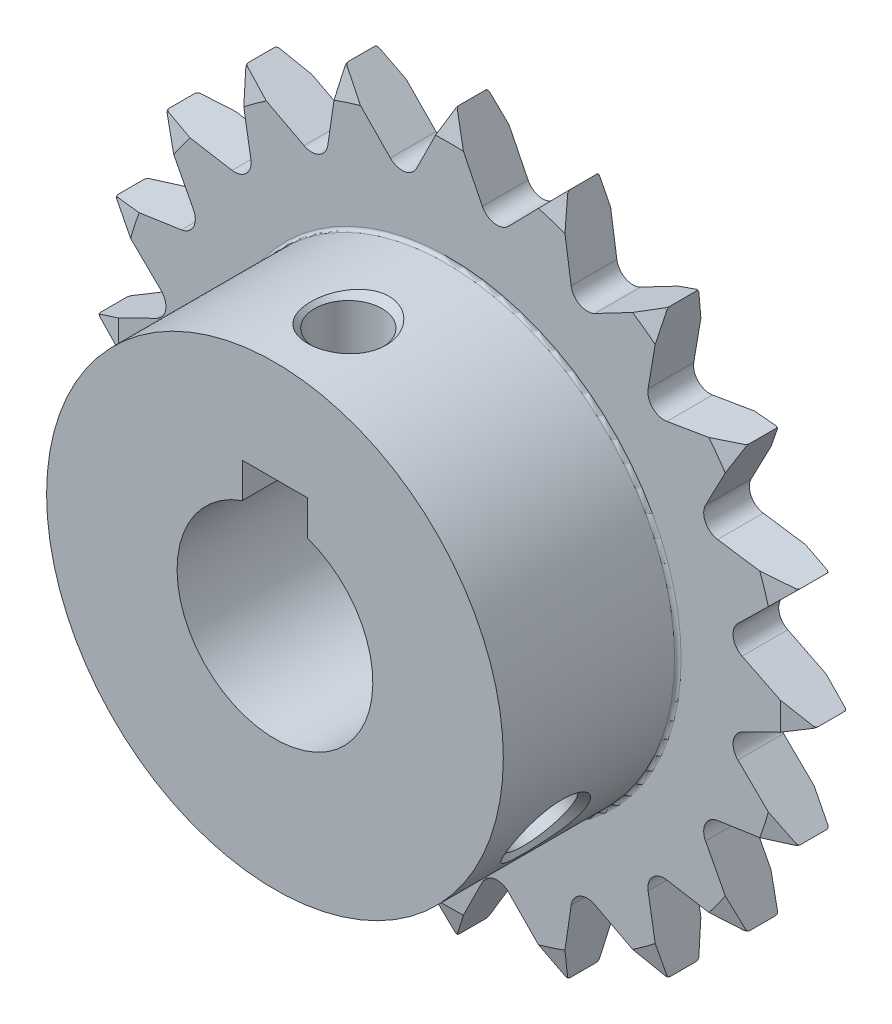
SolidWorks part; units mm, degrees
ref_plane "前视基准面" through (0, 0, 0) normal (0, 0, 1) x (1, 0, 0)
ref_plane "上视基准面" through (0, 0, 0) normal (0, 1, 0) x (1, 0, 0)
ref_plane "右视基准面" through (0, 0, 0) normal (1, 0, 0) x (0, 0, -1)
sketch "草图1" plane through (0, 0, 0) normal (1, 0, 0) x (0, 0, -1)
  line L0 (-15, 6.2) -> (-14.8, 6)
  line L1 (-14.8, 6) -> (-0.2, 6)
  line L2 (-0.2, 6) -> (0, 6.2)
  line L3 (0, 6.2) -> (0, 20.295)
  line L4 (0, 20.295) -> (-0.4171, 21.8518)
  line L5 (-0.6103, 22) -> (-2.1897, 22)
  line L6 (-2.3829, 21.8518) -> (-2.8, 20.295)
  line L7 (-2.8, 20.295) -> (-2.8, 14.2)
  line L8 (-3, 14) -> (-14.8, 14)
  line L9 (-14.8, 14) -> (-15, 13.8)
  line L10 (-15, 13.8) -> (-15, 6.2)
  line L11 (0, 0) -> (-15, 0) construction
  arc A0 (-0.4171, 21.8518) -> (-0.6103, 22) centre (-0.6103, 21.8) ccw
  arc A1 (-2.1897, 22) -> (-2.3829, 21.8518) centre (-2.1897, 21.8) ccw
  arc A2 (-2.8, 14.2) -> (-3, 14) centre (-3, 14.2) cw
revolve "旋转1" add sketch "草图1" angle 360 about L11
sketch "草图2" plane through (0, 0, 0) normal (0, 0, 1) x (1, 0, 0)
  line L0 (-150.3101, -119.3707) -> (151.6954, -119.3707)
  line L1 (151.6954, -119.3707) -> (151.6954, 126.7592)
  line L2 (151.6954, 126.7592) -> (-150.3101, 126.7592)
  line L3 (-150.3101, 126.7592) -> (-150.3101, -119.3707)
  line L4 (-22, 0) -> (-17.938, -2.0157)
  line L5 (-17.6829, -3.6261) -> (-20.9232, -6.7984)
  line L6 (-20.9232, -6.7984) -> (-16.4371, -7.4602)
  line L7 (-15.6969, -8.9129) -> (-17.7984, -12.9313)
  line L8 (-17.7984, -12.9313) -> (-13.3273, -12.1744)
  line L9 (-12.1744, -13.3273) -> (-12.9313, -17.7984)
  line L10 (-12.9313, -17.7984) -> (-8.9129, -15.6969)
  line L11 (-7.4602, -16.4371) -> (-6.7984, -20.9232)
  line L12 (-6.7984, -20.9232) -> (-3.6261, -17.6829)
  line L13 (-2.0157, -17.938) -> (0, -22)
  line L14 (0, -22) -> (2.0157, -17.938)
  line L15 (3.6261, -17.6829) -> (6.7984, -20.9232)
  line L16 (6.7984, -20.9232) -> (7.4602, -16.4371)
  line L17 (8.9129, -15.6969) -> (12.9313, -17.7984)
  line L18 (12.9313, -17.7984) -> (12.1744, -13.3273)
  line L19 (13.3273, -12.1744) -> (17.7984, -12.9313)
  line L20 (17.7984, -12.9313) -> (15.6969, -8.9129)
  line L21 (16.4371, -7.4602) -> (20.9232, -6.7984)
  line L22 (20.9232, -6.7984) -> (17.6829, -3.6261)
  line L23 (17.938, -2.0157) -> (22, 0)
  line L24 (22, 0) -> (17.938, 2.0157)
  line L25 (17.6829, 3.6261) -> (20.9232, 6.7984)
  line L26 (20.9232, 6.7984) -> (16.4371, 7.4602)
  line L27 (15.6969, 8.9129) -> (17.7984, 12.9313)
  line L28 (17.7984, 12.9313) -> (13.3273, 12.1744)
  line L29 (12.1744, 13.3273) -> (12.9313, 17.7984)
  line L30 (12.9313, 17.7984) -> (8.9129, 15.6969)
  line L31 (7.4602, 16.4371) -> (6.7984, 20.9232)
  line L32 (6.7984, 20.9232) -> (3.6261, 17.6829)
  line L33 (2.0157, 17.938) -> (0, 22)
  line L34 (0, 22) -> (-2.0157, 17.938)
  line L35 (-3.6261, 17.6829) -> (-6.7984, 20.9232)
  line L36 (-6.7984, 20.9232) -> (-7.4602, 16.4371)
  line L37 (-8.9129, 15.6969) -> (-12.9313, 17.7984)
  line L38 (-12.9313, 17.7984) -> (-12.1744, 13.3273)
  line L39 (-13.3273, 12.1744) -> (-17.7984, 12.9313)
  line L40 (-17.7984, 12.9313) -> (-15.6969, 8.9129)
  line L41 (-16.4371, 7.4602) -> (-20.9232, 6.7984)
  line L42 (-20.9232, 6.7984) -> (-17.6829, 3.6261)
  line L43 (-17.938, 2.0157) -> (-22, 0)
  arc A0 (-17.938, -2.0157) -> (-17.6829, -3.6261) centre (-18.3825, -2.9115) cw
  arc A1 (-16.4371, -7.4602) -> (-15.6969, -8.9129) centre (-16.5831, -8.4495) cw
  arc A2 (-13.3273, -12.1744) -> (-12.1744, -13.3273) centre (-13.1604, -13.1604) cw
  arc A3 (-8.9129, -15.6969) -> (-7.4602, -16.4371) centre (-8.4495, -16.5831) cw
  arc A4 (-3.6261, -17.6829) -> (-2.0157, -17.938) centre (-2.9115, -18.3825) cw
  arc A5 (2.0157, -17.938) -> (3.6261, -17.6829) centre (2.9115, -18.3825) cw
  arc A6 (7.4602, -16.4371) -> (8.9129, -15.6969) centre (8.4495, -16.5831) cw
  arc A7 (12.1744, -13.3273) -> (13.3273, -12.1744) centre (13.1604, -13.1604) cw
  arc A8 (15.6969, -8.9129) -> (16.4371, -7.4602) centre (16.5831, -8.4495) cw
  arc A9 (17.6829, -3.6261) -> (17.938, -2.0157) centre (18.3825, -2.9115) cw
  arc A10 (17.938, 2.0157) -> (17.6829, 3.6261) centre (18.3825, 2.9115) cw
  arc A11 (16.4371, 7.4602) -> (15.6969, 8.9129) centre (16.5831, 8.4495) cw
  arc A12 (13.3273, 12.1744) -> (12.1744, 13.3273) centre (13.1604, 13.1604) cw
  arc A13 (8.9129, 15.6969) -> (7.4602, 16.4371) centre (8.4495, 16.5831) cw
  arc A14 (3.6261, 17.6829) -> (2.0157, 17.938) centre (2.9115, 18.3825) cw
  arc A15 (-2.0157, 17.938) -> (-3.6261, 17.6829) centre (-2.9115, 18.3825) cw
  arc A16 (-7.4602, 16.4371) -> (-8.9129, 15.6969) centre (-8.4495, 16.5831) cw
  arc A17 (-12.1744, 13.3273) -> (-13.3273, 12.1744) centre (-13.1604, 13.1604) cw
  arc A18 (-15.6969, 8.9129) -> (-16.4371, 7.4602) centre (-16.5831, 8.4495) cw
  arc A19 (-17.6829, 3.6261) -> (-17.938, 2.0157) centre (-18.3825, 2.9115) cw
extrude "切除-拉伸1" cut sketch "草图2" along normal blind 2.8
ref_plane "基准面4" through (0, 0, 9) normal (0, 0, 1) x (1, 0, 0)
sketch "草图3" plane through (0, 0, 9) normal (0, 0, 1) x (1, 0, 0)
  line L0 (0, 1.8) -> (-2.5, 1.8)
  line L1 (-2.5, 1.8) -> (-2.5, 7.8)
  line L2 (-2.5, 7.8) -> (-2.067, 8.233)
  line L3 (-2.067, 8.233) -> (-2.067, 13.567)
  line L4 (-2.067, 13.567) -> (-2.5, 14)
  line L5 (-2.5, 14) -> (-2.5, 20)
  line L6 (-2.5, 20) -> (0, 20)
  line L7 (0, 20) -> (0, 1.8)
  line L8 (0, 14) -> (0, 7.8) construction
revolve "切除-旋转1" cut sketch "草图3" angle 360 about L8
cosmetic thread "装饰螺纹线1" parameters "D1"=5.767, "D2"=5
sketch "草图4" plane through (0, 0, 9) normal (0, 0, 1) x (1, 0, 0)
  line L0 (0, 0) -> (1.25, 2.1651)
  line L1 (1.25, 2.1651) -> (6.4462, -0.8349)
  line L2 (6.4462, -0.8349) -> (6.6046, -1.4264)
  line L3 (6.6046, -1.4264) -> (12.7829, -4.9934)
  line L4 (12.7829, -4.9934) -> (13.3744, -4.8349)
  line L5 (13.3744, -4.8349) -> (18.5705, -7.8349)
  line L6 (18.5705, -7.8349) -> (17.3205, -10)
  line L7 (17.3205, -10) -> (0, 0)
  line L8 (12.1244, -7) -> (5.1962, -3) construction
revolve "切除-旋转2" cut sketch "草图4" angle 360 about L8
cosmetic thread "装饰螺纹线2" parameters "D1"=7.567, "D2"=5
sketch "草图5" plane through (0, 0, 0) normal (0, 0, 1) x (1, 0, 0)
  line L0 (-2, 0) -> (2, 0)
  line L1 (2, 0) -> (2, 7.8)
  line L2 (2, 7.8) -> (-2, 7.8)
  line L3 (-2, 7.8) -> (-2, 0)
extrude "切除-拉伸2" cut sketch "草图5" along normal blind 15
sketch "草图6" plane through (0, 0, 0) normal (0, 1, 0) x (1, 0, 0)
  line L1 (-14.4002, -15) -> (14.6853, -15)
  line L2 (-14.4002, -15) -> (-14.4002, -13.5)
  line L3 (-14.4002, -13.5) -> (14.6853, -13.5)
  line L4 (14.6853, -15) -> (14.6853, -13.5)
  dimension "D1" = 1.5
extrude "切除-拉伸3" cut sketch "草图6" against normal through all and the other way through all
